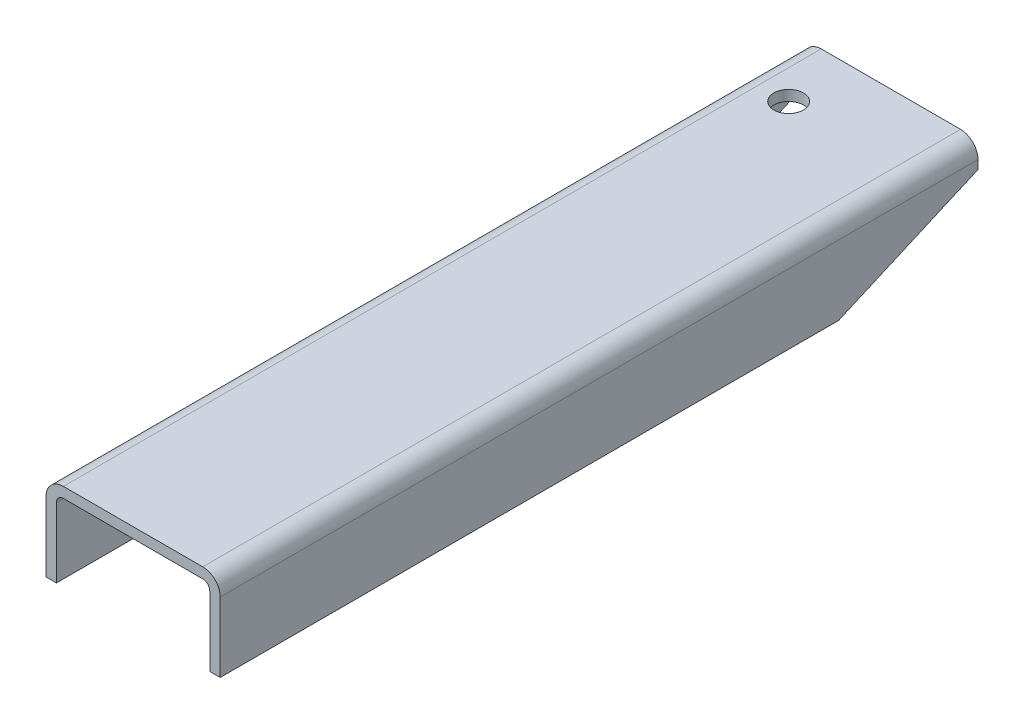
SolidWorks part; units mm, degrees
material "1023 Carbon Steel Plate (SS)"
ref_plane "Front Plane" through (0, 0, 0) normal (0, 0, 1) x (1, 0, 0)
ref_plane "Top Plane" through (0, 0, 0) normal (0, 1, 0) x (1, 0, 0)
ref_plane "Right Plane" through (0, 0, 0) normal (1, 0, 0) x (0, 0, -1)
sketch "Sketch1" plane through (0, 0, 0) normal (0, 0, 1) x (1, 0, 0)
  line L0 (0, 0) -> (0, 40)
  line L1 (10, 50) -> (90, 50)
  line L2 (100, 40) -> (100, 0)
  line L3 (6, 0) -> (6, 40)
  line L4 (10, 44) -> (90, 44)
  line L5 (94, 40) -> (94, 0)
  line L6 (6, 0) -> (0, 0)
  line L7 (100, 0) -> (94, 0)
  arc A0 (90, 50) -> (100, 40) centre (90, 40) cw
  arc A1 (0, 40) -> (10, 50) centre (10, 40) cw
  arc A2 (6, 40) -> (10, 44) centre (10, 40) cw
  arc A3 (90, 44) -> (94, 40) centre (90, 40) cw
  point P7 (100, 50)
  point P10 (0, 50)
  dimension "D4" = 10
  dimension "D1" = 50
  dimension "D2" = 100
  dimension "D3" = 50
  dimension "D5" = 6
extrude "Boss-Extrude1" add sketch "Sketch1" along normal blind 435 contours L7 L5 A3 L4 A2 L3 L6 L0 A1 L1 A0 L2
sketch "Sketch2" plane through (0, 50, 0) normal (0, 1, 0) x (1, 0, 0)
  line L1 (10, -435) -> (90, -435) construction
  line L2 (100, -435) -> (100, 0) construction
  circle A0 centre (26.8, -35.5) radius 8.5
  dimension "D1" = 73.2
  dimension "D2" = 399.5
  dimension "D3" = 17
extrude "Cut-Extrude1" cut sketch "Sketch2" against normal blind 435
sketch "Sketch3" plane through (100, 0, 0) normal (1, 0, 0) x (0, 0, -1)
  line L0 (-80, 0) -> (0, 35)
  line L1 (-435, 0) -> (0, 0) construction
  line L2 (0, 40) -> (0, 0) construction
  line L3 (0, 35) -> (0, 0)
  line L4 (0, 0) -> (-80, 0)
  dimension "D1" = 80
  dimension "D2" = 35
extrude "Cut-Extrude2" cut sketch "Sketch3" against normal blind 435
